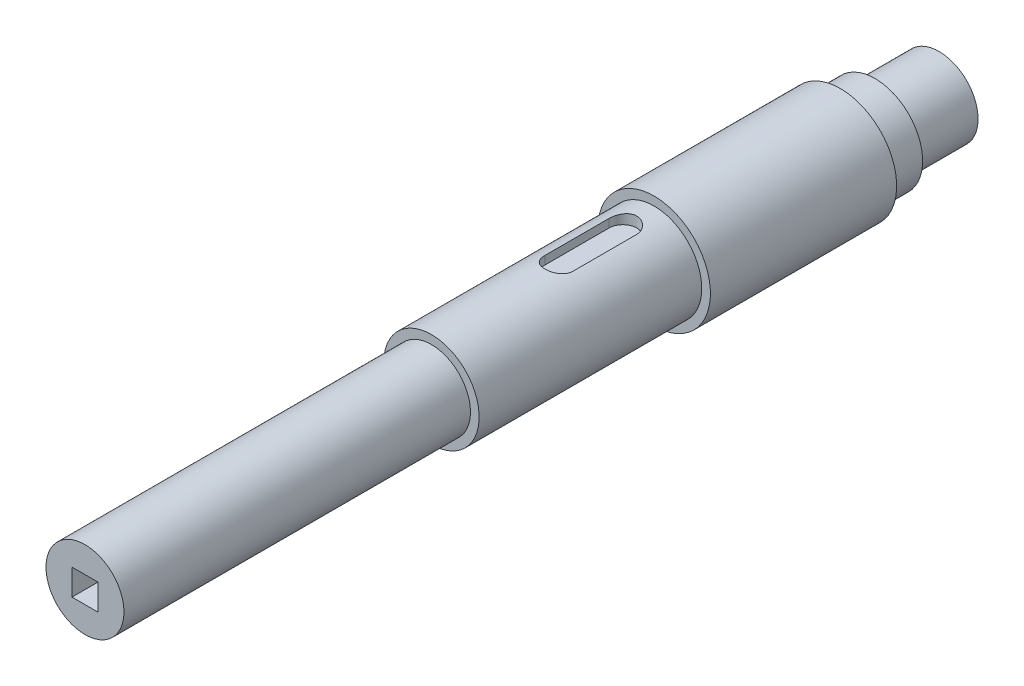
SolidWorks part; units mm, degrees
ref_plane "前视基准面" through (0, 0, 0) normal (0, 0, 1) x (1, 0, 0)
ref_plane "上视基准面" through (0, 0, 0) normal (0, 1, 0) x (1, 0, 0)
ref_plane "右视基准面" through (0, 0, 0) normal (1, 0, 0) x (0, 0, -1)
sketch "草图1" plane through (0, 0, 0) normal (0, 1, 0) x (1, 0, 0)
  line L0 (0, 0) -> (0, -74086.4682) construction
  line L1 (0, 200) -> (-22.5, 200)
  line L2 (-22.5, 200) -> (-22.5, 163)
  line L3 (-22.5, 163) -> (-27.5, 163)
  line L4 (-27.5, 163) -> (-27.5, 143)
  line L5 (-27.5, -93) -> (-22.5, -93)
  line L6 (-22.5, -93) -> (-22.5, -293)
  line L7 (-22.5, -293) -> (0, -293)
  line L8 (0, 200) -> (0, -293)
  line L9 (-27.5, 35.5) -> (-32.5, 35.5)
  line L10 (-32.5, 35.5) -> (-32.5, 143)
  line L11 (-32.5, 143) -> (-27.5, 143)
  line L12 (-27.5, 35.5) -> (-27.5, -93)
  dimension "D1" = 55
  dimension "D2" = 45
  dimension "D3" = 256
  dimension "D4" = 37
  dimension "D5" = 200
  dimension "D6" = 200
  dimension "D7" = 128.5
  dimension "D8" = 65
  dimension "D9" = 20
revolve "旋转1" add sketch "草图1" angle 360 about L0
sketch "草图2" plane through (0, 0, -200) normal (0, 0, -1) x (-1, 0, 0)
  line L1 (7.5, 7.5) -> (-7.5, 7.5)
  line L2 (7.5, 7.5) -> (7.5, -7.5)
  line L3 (7.5, -7.5) -> (-7.5, -7.5)
  line L4 (-7.5, 7.5) -> (-7.5, -7.5)
  line L5 (7.5, 7.5) -> (-7.5, -7.5) construction
  line L6 (7.5, -7.5) -> (-7.5, 7.5) construction
  point P0 (0, 0)
  dimension "D1" = 15
extrude "切除-拉伸1" cut sketch "草图2" against normal through all
chamfer "倒角1" distance 3 angle 60 4 edges at (7.5, 0, -200) (0, 7.5, -200) (-7.5, 0, -200) (0, -7.5, -200)
ref_plane "基准面1" through (0, 27.5, 0) normal (0, 1, 0) x (1, 0, 0)
sketch "草图3" plane through (0, 27.5, 0) normal (0, 1, 0) x (1, 0, 0)
  line L0 (0, -19.5) -> (0, 17.5) construction
  line L1 (-8, -19.5) -> (-8, 17.5)
  line L2 (8, -19.5) -> (8, 17.5)
  line L4 (-27.5, 35.5) -> (27.5, 35.5) construction
  arc A0 (-8, -19.5) -> (8, -19.5) centre (0, -19.5) ccw
  arc A1 (8, 17.5) -> (-8, 17.5) centre (0, 17.5) ccw
  point P2 (0, -1)
  point P10 (-8, -1)
  dimension "D1" = 10
  dimension "D3" = 53
  dimension "D2" = 16
extrude "切除-拉伸2" cut sketch "草图3" against normal blind 6
